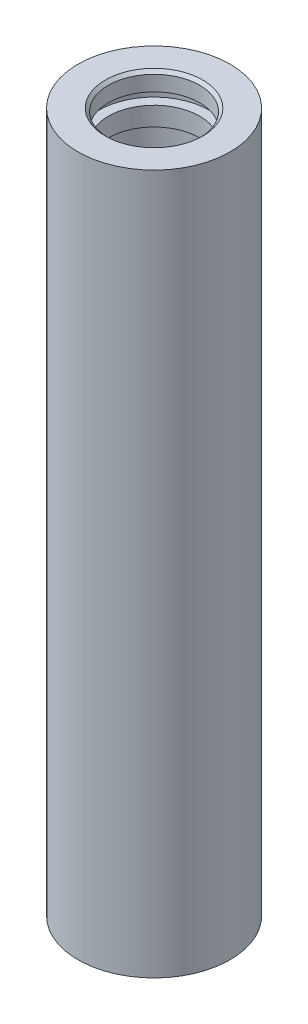
SolidWorks part; units mm, degrees
material "A3"
ref_plane "前视基准面" through (0, 0, 0) normal (0, 0, 1) x (1, 0, 0)
ref_plane "上视基准面" through (0, 0, 0) normal (0, 1, 0) x (1, 0, 0)
ref_plane "右视基准面" through (0, 0, 0) normal (1, 0, 0) x (0, 0, -1)
sketch "草图1" plane through (0, 0, 0) normal (0, 0, 1) x (1, 0, 0)
  line L0 (0, 0) -> (0, 230) construction
  line L1 (8.0822, 0) -> (25, 0)
  line L2 (25, 0) -> (25, 230)
  line L3 (25, 230) -> (15, 230)
  line L4 (15, 230) -> (15, 224)
  line L5 (15, 224) -> (18.27, 224)
  line L6 (18.27, 224) -> (18.27, 220.2)
  line L7 (18.27, 220.2) -> (15, 220.2)
  line L8 (15, 220.2) -> (15, 214)
  line L9 (15, 214) -> (18, 214)
  line L10 (18, 214) -> (18, 16)
  line L11 (25, 115) -> (16.165, 115) construction
  line L12 (15, 16) -> (18, 16)
  line L13 (15, 9.8) -> (15, 16)
  line L14 (18.27, 9.8) -> (15, 9.8)
  line L15 (18.27, 6) -> (18.27, 9.8)
  line L16 (15, 6) -> (18.27, 6)
  line L17 (15, 0) -> (15, 6)
  line L18 (25, 0) -> (15, 0)
  point P18 (18, 115)
  dimension "D1" = 230
  dimension "D2" = 50
  dimension "D3" = 30
  dimension "D4" = 36
  dimension "D5" = 6
  dimension "D6" = 10
  dimension "D7" = 3.8
  dimension "D8" = 3.27
revolve "旋转1" add sketch "草图1" angle 360 about L0
chamfer "倒角1" distance 1 angle 45 2 edges at (0, 0, -15) (0, 230, -15)
